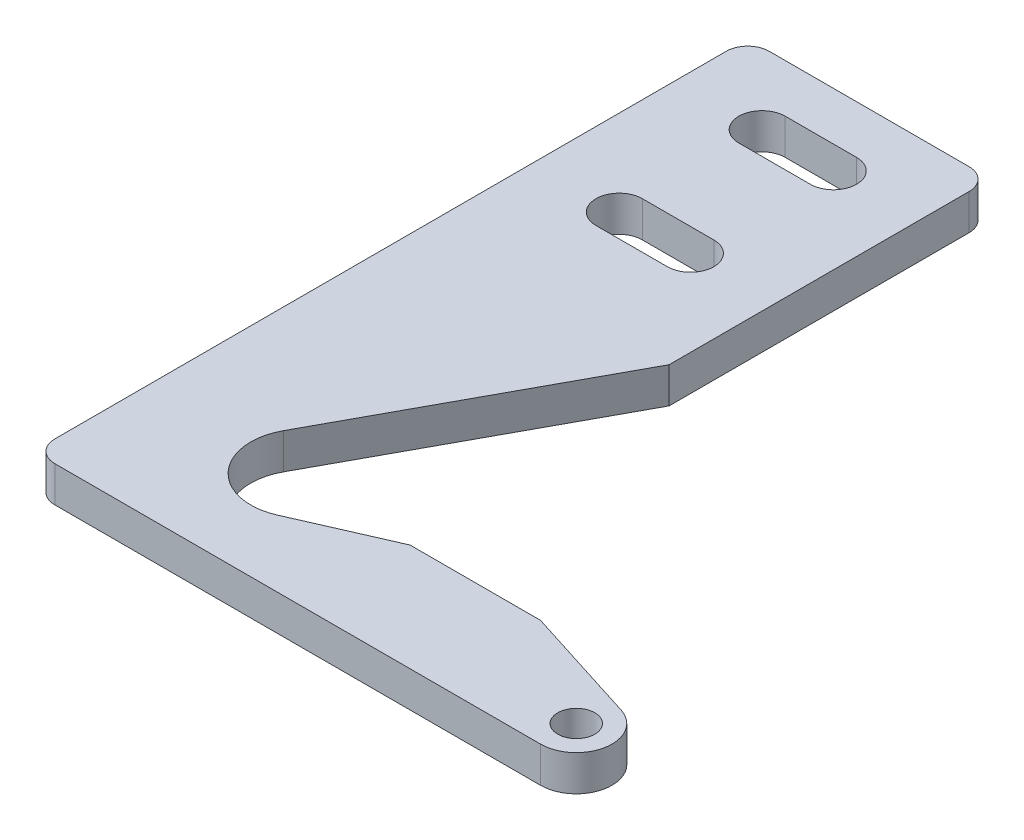
from build123d import *

# Parameters (mm, degrees)
SKETCH1_R           = 2.6
BOSS_EXTRUDE1_DEPTH = 5
FILLET1_R           = 3


with BuildPart() as part:
    # Sketch1 → Boss-Extrude1 (new body)
    with BuildSketch(Plane(origin=(0, 0, 0), x_dir=(1, 0, 0), z_dir=(0, 1, 0))):
        with BuildLine():
            Line((-17, 10), (-17, -90))
            Line((-17, -90), (54, -90))
            ThreePointArc((54, -90), (58.941222292, -85.764409749), (55.510847396, -80.233728906))
            Line((55.510847396, -80.233728906), (39, -75))
            Line((39, -75), (20.726086957, -75))
            Line((20.726086957, -75), (7.79590612, -80.661902004))
            ThreePointArc((7.79590612, -80.661902004), (-0.909612834, -78.829253465), (-2, -70))
            Line((-2, -70), (17, -35))
            Line((17, -35), (17, 10))
            Line((17, 10), (-17, 10))
        make_face()
        with Locations(Location((54, -85, 0), (0, 0, 270))):
            Circle(SKETCH1_R, mode=Mode.SUBTRACT)
        with BuildLine():
            Line((5, -3.25), (-5, -3.25))
            ThreePointArc((-5, -3.25), (-8.25, 0), (-5, 3.25))
            Line((-5, 3.25), (5, 3.25))
            ThreePointArc((5, 3.25), (8.25, 0), (5, -3.25))
        make_face(mode=Mode.SUBTRACT)
        with BuildLine():
            Line((5, -23.25), (-5, -23.25))
            ThreePointArc((-5, -23.25), (-8.25, -20), (-5, -16.75))
            Line((-5, -16.75), (5, -16.75))
            ThreePointArc((5, -16.75), (8.25, -20), (5, -23.25))
        make_face(mode=Mode.SUBTRACT)
    extrude(amount=BOSS_EXTRUDE1_DEPTH)

    # Fillet1
    fillet1_edges = [part.edges().sort_by_distance(p)[0] for p in [
        (17, 2.5, -10),
        (-17, 2.5, 90),
        (-17, 2.5, -10),
    ]]
    fillet(fillet1_edges, radius=FILLET1_R)


solid = part.part
